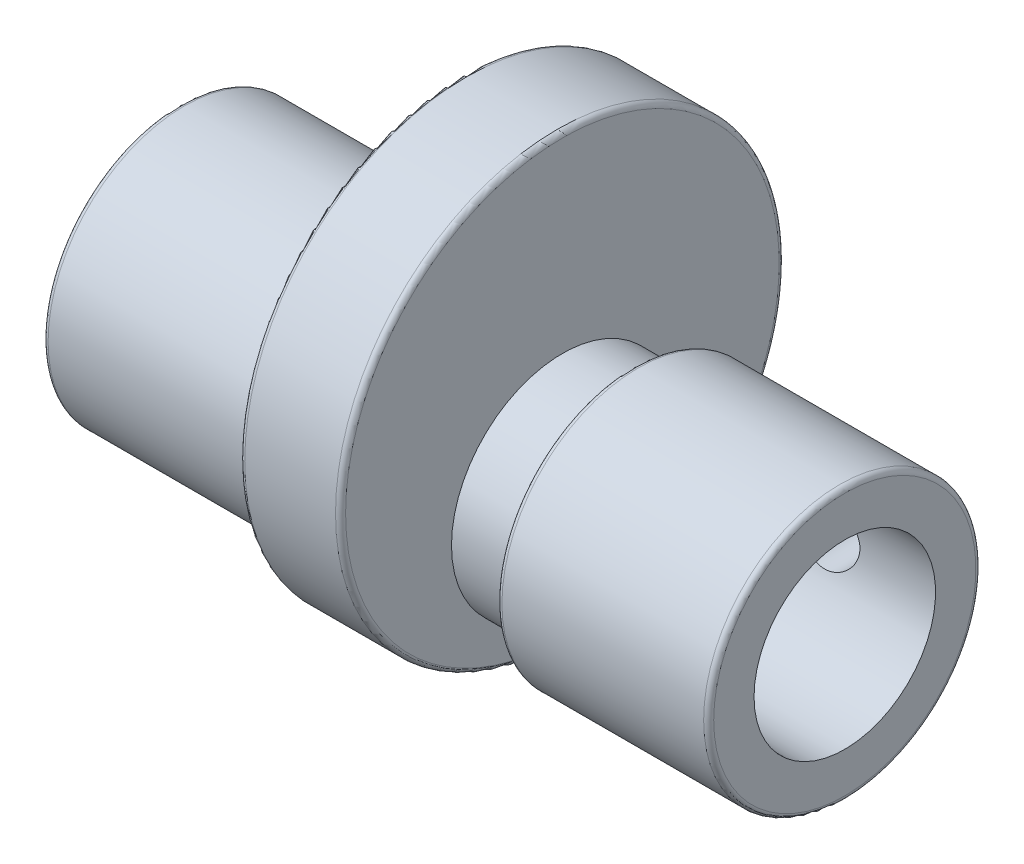
from build123d import *

# Parameters (mm, degrees)
SKETCH2_R           = 22
BOSS_EXTRUDE1_DEPTH = 5
SKETCH3_R           = 8
CUT_EXTRUDE1_DEPTH  = 13
FILLET1_R           = 0.5
SKETCH4_R           = 3
CUT_EXTRUDE2_DEPTH  = 26


with BuildPart() as part:
    # Sketch1 → Revolve1 (revolve)
    with BuildSketch(Plane.XY, mode=Mode.PRIVATE) as revolve1_sk:
        Polygon((0, 9), (0, 13.5), (21, 13.5), (21, 11), (45, 11), (45, 13.5), (66, 13.5), (66, 9), (51, 9), (51, 8), (15, 8), (15, 9), align=None)
    revolve(revolve1_sk.sketch.rotate(Axis((0, 0, 0), (1, 0, 0)), 90), axis=Axis((0, 0, 0), (1, 0, 0)))

    # Sketch2 → Boss-Extrude1 (add, symmetric)
    with BuildSketch(Plane.ZY.offset(-33)):
        with Locations((0, 8)):
            Circle(SKETCH2_R)
    extrude(amount=BOSS_EXTRUDE1_DEPTH, both=True)

    # Sketch3 → Cut-Extrude1 (cut, symmetric)
    with BuildSketch(Plane(origin=(38, 0, 0), x_dir=(0, 0, -1), z_dir=(1, 0, 0))):
        with Locations(Location((0, 0, 0), (0, 0, 180))):
            Circle(SKETCH3_R)
    extrude(amount=CUT_EXTRUDE1_DEPTH, both=True, mode=Mode.SUBTRACT)

    # Fillet1
    fillet1_edges = [part.edges().sort_by_distance(p)[0] for p in [
        (66, 0, -13.5),
        (45, 0, -13.5),
        (21, 0, -13.5),
        (0, 0, -13.5),
        (28, 8, -22),
        (38, 8, -22),
    ]]
    fillet(fillet1_edges, radius=FILLET1_R)

    # Sketch4 → Cut-Extrude2 (cut)
    with BuildSketch(Plane.XY):
        with Locations((55.5, 0)):
            Circle(SKETCH4_R)
    extrude(amount=-CUT_EXTRUDE2_DEPTH, mode=Mode.SUBTRACT)


solid = part.part
